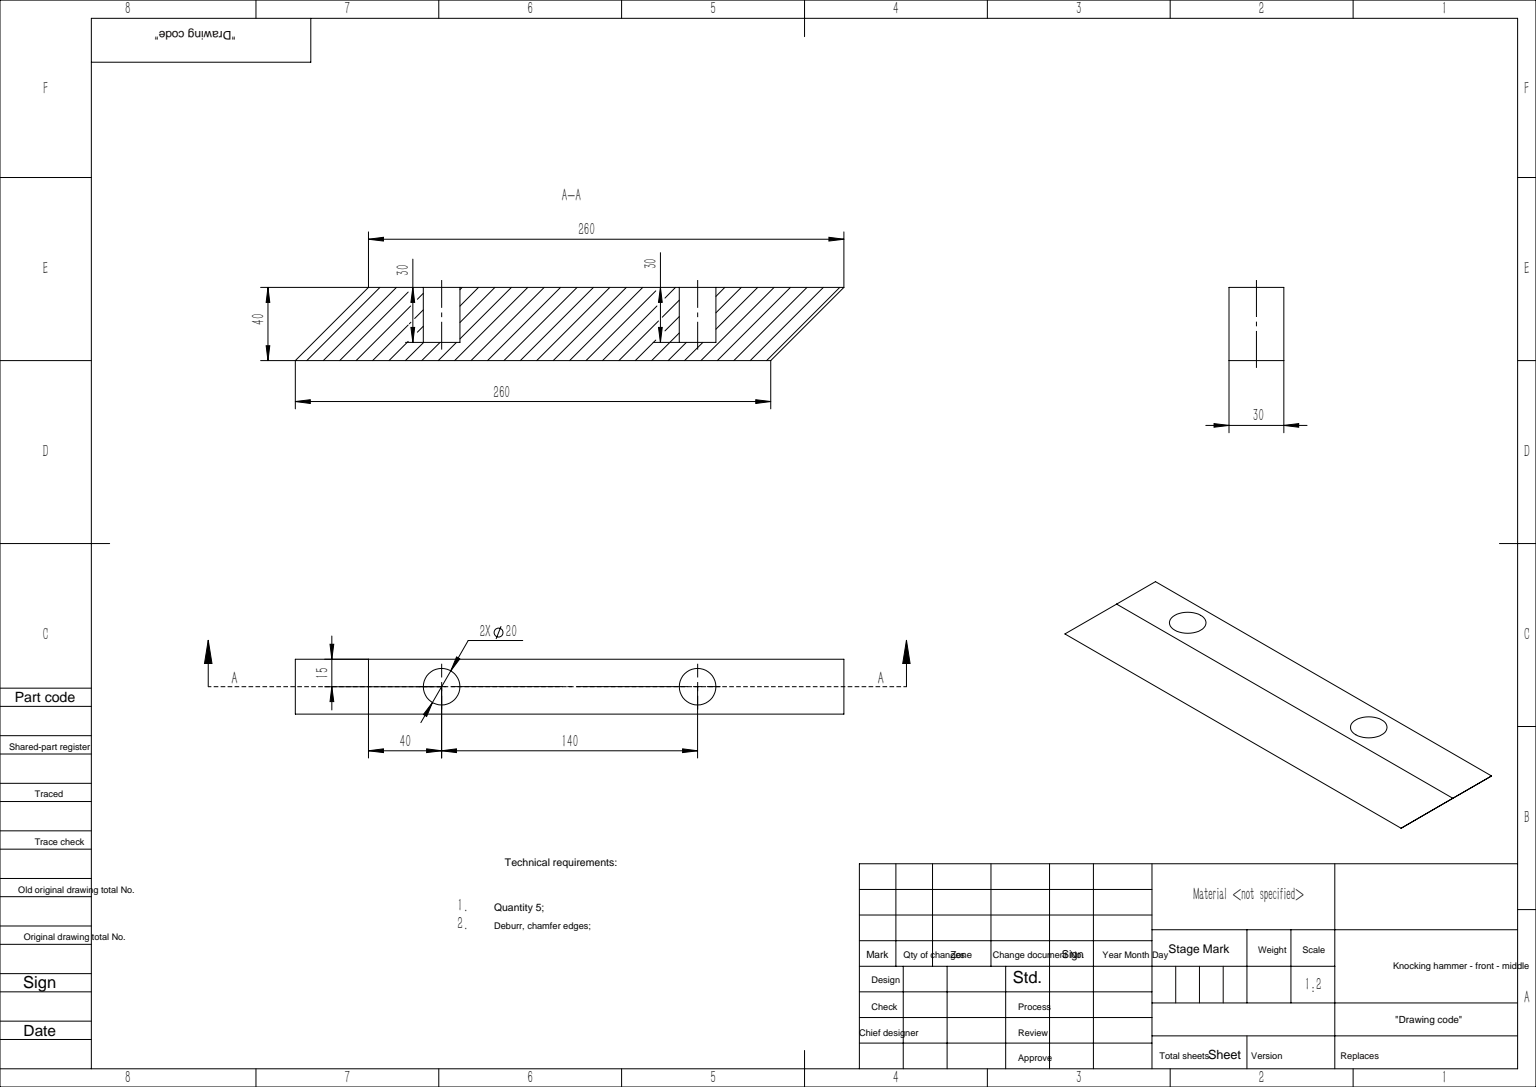
from build123d import *

# Parameters (mm, degrees)
SKETCH_1_W          = 270
SKETCH_1_H          = 30
EXTRUDE_1_DEPTH     = 40
SKETCH_2_R          = 10
CUT_EXTRUDE_2_DEPTH = 30
SKETCH_3_W          = 30
SKETCH_3_H          = 40
EXTRUDE_2_DEPTH     = 15
CUT_EXTRUDE_3_DEPTH = 159.113883008
SKETCH_5_W          = 30
SKETCH_5_H          = 40
EXTRUDE_3_DEPTH     = 15
CUT_EXTRUDE_4_DEPTH = 159.113883008


with BuildPart() as part:
    # 草图1 → 凸台-拉伸1 (new body)
    with BuildSketch(Plane(origin=(0, 0, 0), x_dir=(1, 0, 0), z_dir=(0, 1, 0))):
        Rectangle(SKETCH_1_W, SKETCH_1_H)
    extrude(amount=EXTRUDE_1_DEPTH)

    # 草图2 → 切除-拉伸2 (cut)
    with BuildSketch(Plane(origin=(0, 40, 0), x_dir=(1, 0, 0), z_dir=(0, 1, 0))):
        with Locations(Location((70, 0, 0), (0, 0, 270))):
            Circle(SKETCH_2_R)
        with Locations(Location((-70, 0, 0), (0, 0, 90))):
            Circle(SKETCH_2_R)
    extrude(amount=-CUT_EXTRUDE_2_DEPTH, mode=Mode.SUBTRACT)

    # 草图3 → 凸台-拉伸2 (add)
    with BuildSketch(Plane(origin=(135, 0, 0), x_dir=(0, 0, -1), z_dir=(1, 0, 0))):
        with Locations((0, 20)):
            Rectangle(SKETCH_3_W, SKETCH_3_H)
    extrude(amount=EXTRUDE_2_DEPTH)

    # 草图4 → 切除-拉伸3 (cut, through all)
    with BuildSketch(Plane.XY.offset(15)):
        Polygon((150, 40), (110, 0), (150, 0), align=None)
    extrude(amount=-CUT_EXTRUDE_3_DEPTH, mode=Mode.SUBTRACT)

    # 草图5 → 凸台-拉伸3 (add)
    with BuildSketch(Plane.ZY.offset(135)):
        with Locations((0, 20)):
            Rectangle(SKETCH_5_W, SKETCH_5_H)
    extrude(amount=EXTRUDE_3_DEPTH)

    # 草图6 → 切除-拉伸4 (cut, through all)
    with BuildSketch(Plane.XY.offset(15)):
        Polygon((-150, 0), (-110, 40), (-150, 40), align=None)
    extrude(amount=-CUT_EXTRUDE_4_DEPTH, mode=Mode.SUBTRACT)


solid = part.part
